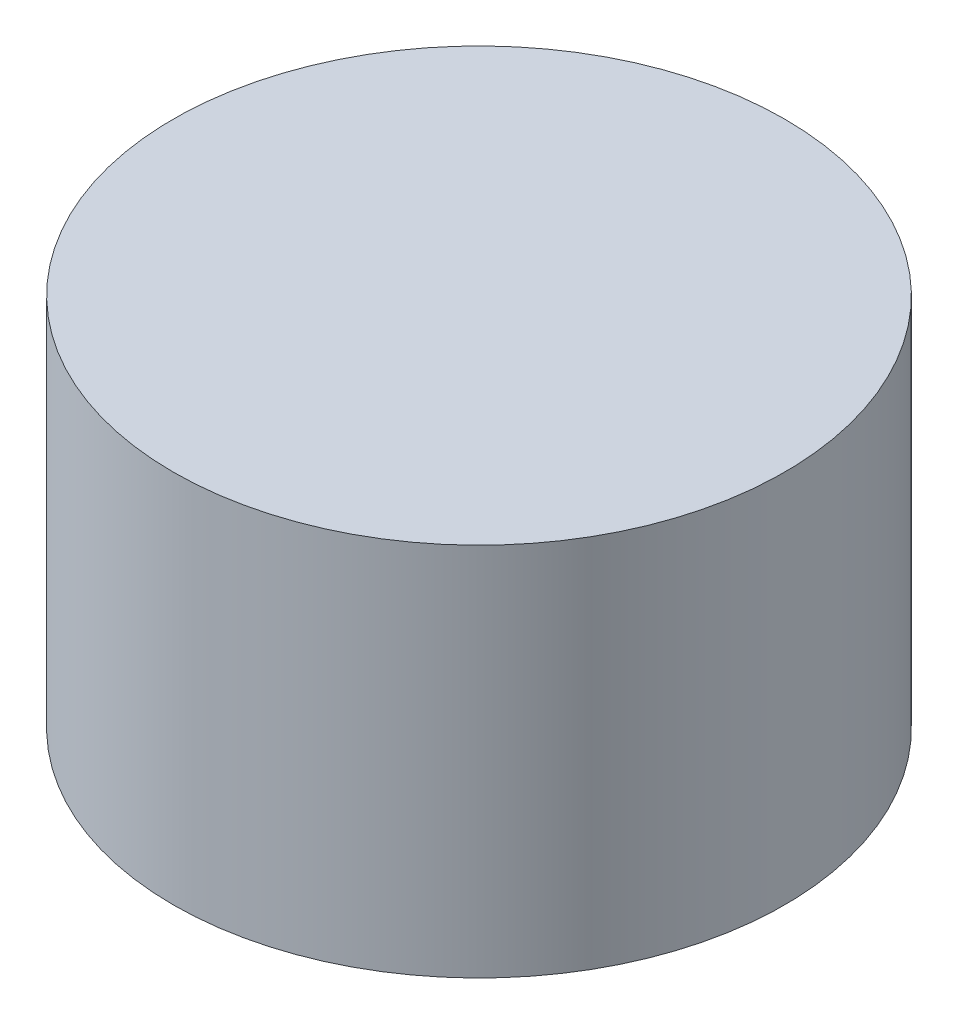
SolidWorks part; units mm, degrees
ref_plane "前视基准面" through (0, 0, 0) normal (0, 0, 1) x (1, 0, 0)
ref_plane "上视基准面" through (0, 0, 0) normal (0, 1, 0) x (1, 0, 0)
ref_plane "右视基准面" through (0, 0, 0) normal (1, 0, 0) x (0, 0, -1)
sketch "草图1" plane through (0, 0, 0) normal (0, 1, 0) x (1, 0, 0)
  circle A0 centre (0, 0) radius 24.4702
extrude "凸台-拉伸1" add sketch "草图1" along normal blind 30
